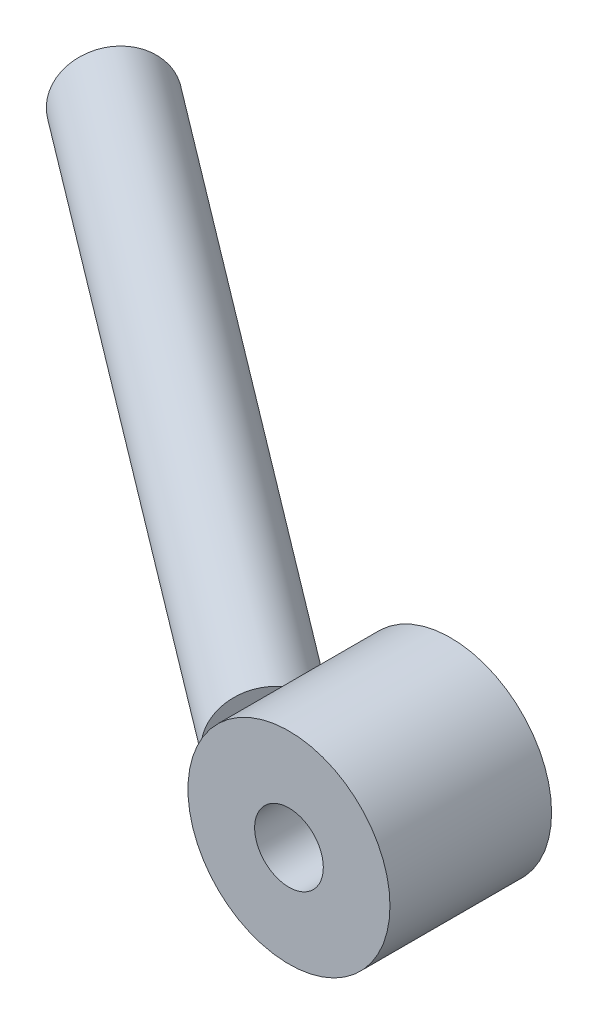
SolidWorks part; units mm, degrees
material "Q235B"
ref_plane "Front" through (0, 0, 0) normal (0, 0, 1) x (1, 0, 0)
ref_plane "Top" through (0, 0, 0) normal (0, 1, 0) x (1, 0, 0)
ref_plane "Right" through (0, 0, 0) normal (1, 0, 0) x (0, 0, -1)
sketch "Sketch1" plane through (0, 0, 0) normal (0, 0, 1) x (1, 0, 0)
  circle A0 centre (0, 0) radius 12.5
  dimension "D1" = 25
extrude "Boss-Extrude1" add sketch "Sketch1" along normal mid plane 20
hole_wizard "M10 Tapped Hole1" positions "Sketch3" profile "Sketch4" tap size "M10" standard "GB" end condition up to next
sketch "Sketch3" plane through (0, 0, 10) normal (0, 0, 1) x (1, 0, 0)
  point P2 (0, 0)
sketch "Sketch4" plane through (0, 0, 10) normal (1, 0, 0) x (0, -1, 0)
  line L0 (0, 0) -> (0, 20)
  line L1 (0, 20) -> (4.25, 20)
  line L2 (4.25, 20) -> (4.25, 0)
  line L5 (4.25, 0) -> (0, 0)
  line L11 (0, -6.35) -> (0, 107.95) construction
  dimension "通孔螺纹孔钻头直径" = 8.5
  dimension "通孔螺纹孔钻头深度" = 20
cosmetic thread "Cosmetic Thread1"
sketch "Sketch5" plane through (0, 0, 0) normal (0, 1, 0) x (1, 0, 0)
  line L0 (-12.5, 0) -> (-92.2947, 60.2727)
  line L1 (-12.5, 10) -> (-12.5, -10) construction
  line L2 (-92.2947, 60.2727) -> (-88.6784, 65.0604)
  line L3 (-88.6784, 65.0604) -> (-8.8836, 4.7877)
  line L4 (-12.5, 0) -> (-8.8836, 4.7877)
  dimension "D1" = 6
  dimension "D2" = 100
revolve "Revolve1" add sketch "Sketch5" angle 360 about L0
chamfer "Chamfer1" distance 2 angle 45 1 edges at (-88.6784, 0, -65.0604)
equation "\"零件重量\"= IIF ( \"SW-质量\" > 100 , int ( \"SW-质量\" ) , \"SW-质量\" )"
